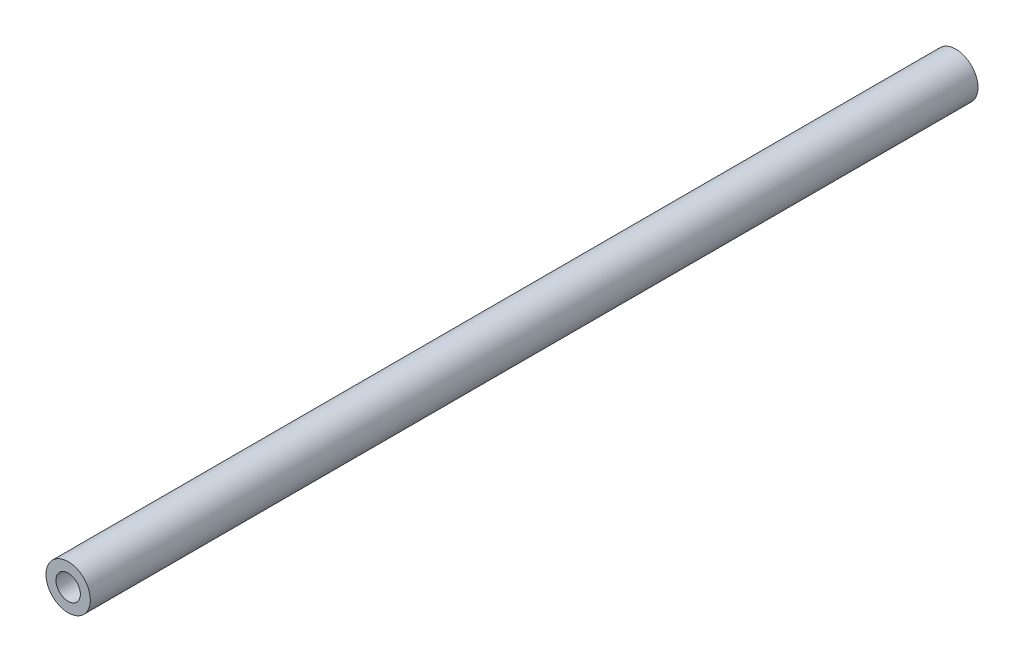
SolidWorks part; units mm, degrees
ref_plane "Front" through (0, 0, 0) normal (0, 0, 1) x (1, 0, 0)
ref_plane "Top" through (0, 0, 0) normal (0, 1, 0) x (1, 0, 0)
ref_plane "Right" through (0, 0, 0) normal (1, 0, 0) x (0, 0, -1)
sketch "Sketch1" plane through (0, 0, 0) normal (0, 0, 1) x (1, 0, 0)
  circle A0 centre (0, 0) radius 3
  dimension "D1" = 6
extrude "Boss-Extrude1" add sketch "Sketch1" along normal mid plane 120
hole_wizard "M4 Tapped Hole1" positions "Sketch3" profile "Sketch2" tap size "M4" standard "Gb"
sketch "Sketch3" plane through (0, 0, 60) normal (0, 0, 1) x (1, 0, 0)
  point P0 (0, 0)
sketch "Sketch2" plane through (0, 0, 60) normal (1, 0, 0) x (0, -1, 0)
  line L0 (0, 0) -> (0, 11.0914)
  line L1 (0, 11.0914) -> (1.65, 10.1)
  line L2 (1.65, 10.1) -> (1.65, 0)
  line L5 (1.65, 0) -> (0, 0)
  line L10 (0, 11.0914) -> (-1.65, 10.1) construction
  line L11 (0, -6.35) -> (0, 107.95) construction
  dimension "螺纹孔钻头直径" = 3.3
  dimension "螺纹孔钻头深度" = 10.1
  dimension "导头角度" = 118
cosmetic thread "Cosmetic Thread1"
hole_wizard "M4 Tapped Hole2" positions "Sketch5" profile "Sketch4" tap size "M4" standard "Gb"
sketch "Sketch5" plane through (0, 0, -60) normal (0, 0, -1) x (-1, 0, 0)
  point P0 (0, 0)
sketch "Sketch4" plane through (0, 0, -60) normal (1, 0, 0) x (0, 1, 0)
  line L0 (0, 0) -> (0, 11.0914)
  line L1 (0, 11.0914) -> (1.65, 10.1)
  line L2 (1.65, 10.1) -> (1.65, 0)
  line L5 (1.65, 0) -> (0, 0)
  line L10 (0, 11.0914) -> (-1.65, 10.1) construction
  line L11 (0, -6.35) -> (0, 107.95) construction
  dimension "螺纹孔钻头直径" = 3.3
  dimension "螺纹孔钻头深度" = 10.1
  dimension "导头角度" = 118
cosmetic thread "Cosmetic Thread2"
